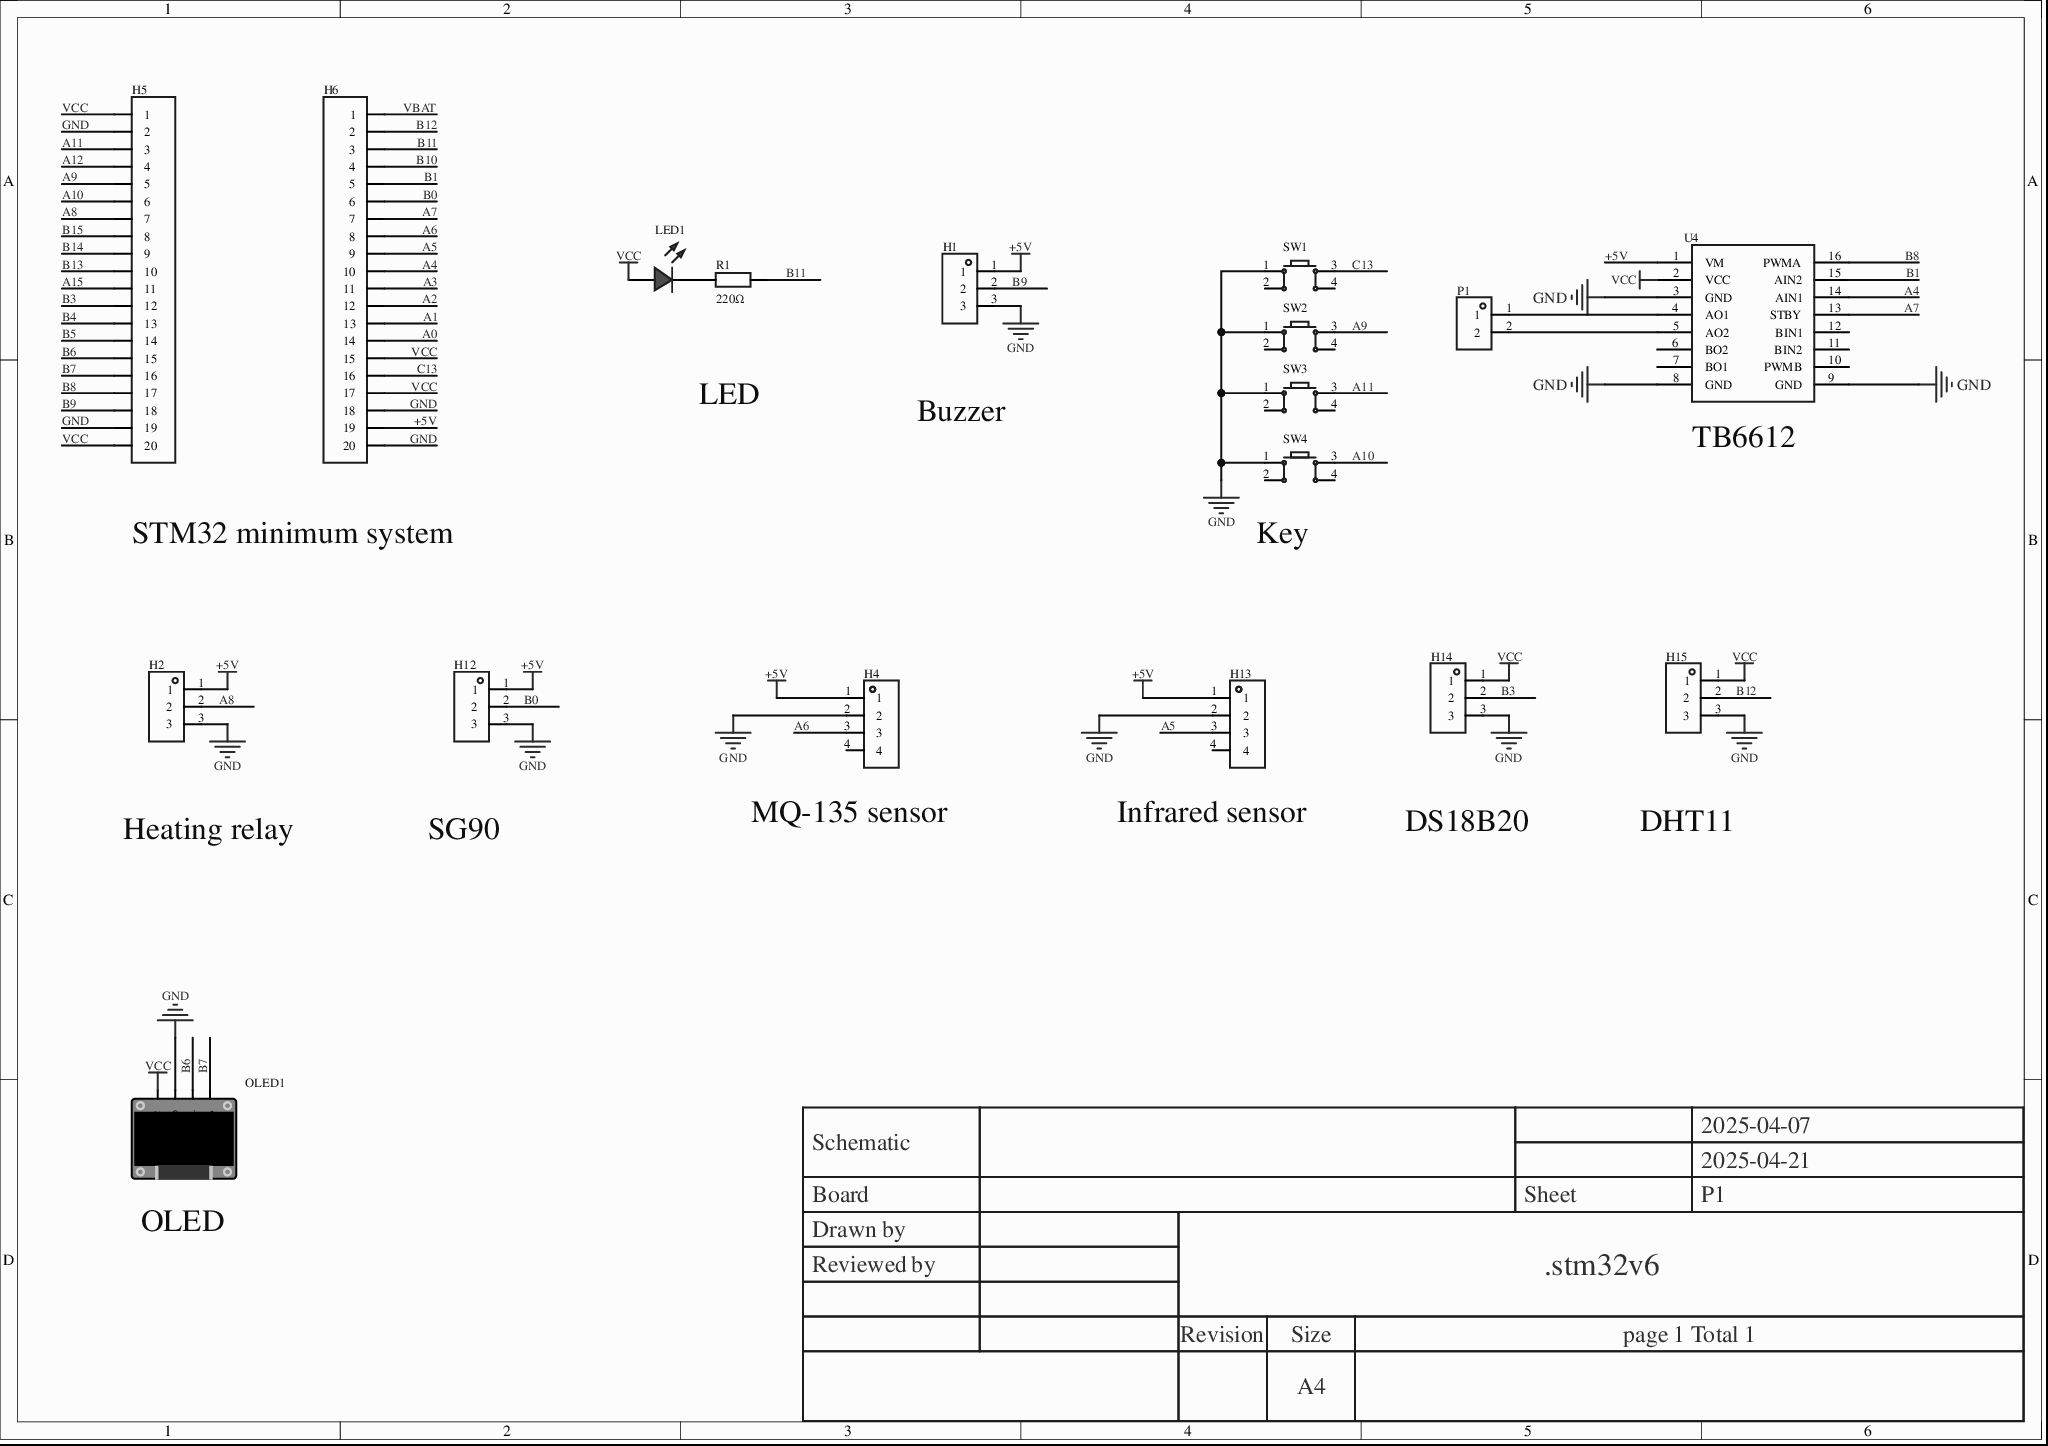
[diagram p0: MISC49946-3.schdoc]
# Altium project MISC49946-2.PrjPcb
1 sheet, 18 parts. Net scope: global (net labels, ports and power ports of the same name join across sheets).
Board file: MISC49946.pcbdoc

## Sheet MISC49946-3.schdoc
size 297 x 209 mm; Version: V1.0; @Project Name: MISC49946; @Page Count: 1; @Update Date: 2026-05-06; @Create Date: 2026-05-06; @Schematic Name: MISC49946; @Page No: 1; @Create Time: 23:22:16; @Update Time: 17:32:40; @Board Name: MISC49946

### Parts
H1  (no value)  [HDR-TH_3P-P2.54-V-F]
H2  (no value)  [HDR-TH_3P-P2.54-V-F]
H4  (no value)  [HDR-TH_4P-P2.54-V-F]
H5  (no value)  [HDR-TH_20P-P2.54-V-F]
H6  (no value)  [HDR-TH_20P-P2.54-V-F]
H12  (no value)  [HDR-TH_3P-P2.54-V-F]
H13  (no value)  [HDR-TH_4P-P2.54-V-F]
H14  (no value)  [HDR-TH_3P-P2.54-V-F]
H15  (no value)  [HDR-TH_3P-P2.54-V-F]
LED1  (no value)  [LED_TH-3mm]
OLED1  (no value)  [0.96OLED_4P]
P1  KF301-2P terminal block  [CONN-TH_XY301V-A-5.0-2P]  (value not drawn)
R1  220Ω  [Res_1/8W]
SW1  (no value)  [SW-TH_4P-L6.0-W6.0-P4.50-LS6.5]
SW2  (no value)  [SW-TH_4P-L6.0-W6.0-P4.50-LS6.5]
SW3  (no value)  [SW-TH_4P-L6.0-W6.0-P4.50-LS6.5]
SW4  (no value)  [SW-TH_4P-L6.0-W6.0-P4.50-LS6.5]
U4  (no value)  [tb6612]

### Nets
+5V: H1.1 H2.1 H4.1 H6.19 H12.1 H13.1 U4.1(VM)
GND: H1.3 H2.3 H4.2 H5.2 H5.19 H6.18 H6.20 H12.3 H13.2 H14.3 H15.3 OLED1.2(GND) SW1.1 SW2.1 SW3.1 SW4.1 U4.3(GND) U4.8(GND) U4.9(GND)
VCC: H5.1 H5.20 H6.15 H6.17 H14.1 H15.1 LED1.1(C) OLED1.1(VCC) U4.2(VCC)
A0: H6.14
A1: H6.13
A2: H6.12
A3: H6.11
A4: H6.10 U4.14(AIN1)
A5: H6.9 H13.3
A6: H4.3 H6.8
A7: H6.7 U4.13(STBY)
A8: H2.2 H5.7
A9: H5.5 SW2.3
A10: H5.6 SW4.3
A11: H5.3 SW3.3
A12: H5.4
A15: H5.11
B0: H6.6 H12.2
B1: H6.5 U4.15(AIN2)
B3: H5.12 H14.2
B4: H5.13
B5: H5.14
B6: H5.15 OLED1.3(SCL)
B7: H5.16 OLED1.4(SDA)
B8: H5.17 U4.16(PWMA)
B9: H1.2 H5.18
B10: H6.4
B11: H6.3 R1.2
B12: H6.2 H15.2
B13: H5.10
B14: H5.9
B15: H5.8
C13: H6.16 SW1.3
VBAT: H6.1
NetLED1_2: LED1.2(A) R1.1
NetP1_1: P1.1 U4.4(AO1)
NetP1_2: P1.2 U4.5(AO2)

Not connected (* = marked no-connect by the designer): H4 4; H13 4; SW1 2 4; SW2 2 4; SW3 2 4; SW4 2 4; U4 6(BO2) 7(BO1) 10(PWMB) 11(BIN2) 12(BIN1)

### Notes on the sheet
- LED
- Buzzer
- (near U4) TB6612
- STM32 minimum system
- (near SW4) Key
- Heating relay
- SG90
- (near H4) MQ-135 sensor
- (near H13) Infrared sensor
- DS18B20
- DHT11
- 串口：
  无通信模块
  GPIO:
  LED灯	PB11
  蜂鸣器  PB9
  按键：	PC13，PA9，PA11，PA10
  加热继电器 PA8
  SG90舵机 PB0
  MQ135空气质量传感器 AO口不接，DO接PA6
  红外AO不接，DO接PA5
  DS18B20   PB3
  DHT11    PB12
  TB6612FNG电机驱动 AO1接有刷小马达+风扇叶正极，AO2接负，PWMA接PB8，AIN2接PB1，AIN1接PA4，STBY接PA7
  IIC:
  0.96英寸OLED显示屏	SDA接PB7 ，SCL接PB6
- OLED
- 2025-04-07
- Schematic
- Board
- Sheet
- 2025-04-21
- P1
- Drawn by
- Reviewed by
- .stm32v6
- Revision
- Size
- A4
- page 1 Total 1

### Library data of the parts
H1 H2 H12 H14 H15 = HDR-F_2.54_1x3P: Symbol: PM254V-11-03-H85; 3D Model: f3b3cc5aae9641bf9e56fc160cef875b; 3D Model Transform: 299.9994,100,0,0,0,0,0,0,-118.11; ConvertToPcb: yes; ModelName: HDR2.54-F-LI-1X3P; Device: HDR-F_2.54_1x3P; Supplier Part: C541850; Supplier Footprint: 插件; FootprintName: HDR-TH_3P-P2.54-V-F; AddInBom: yes
H4 = HDR-F_2.54_1x4P: Symbol: 2.54-1*4P female; ConvertToPcb: yes; ModelId: d187812051054f85879fcaa51a310d8e0819f05c4eef4c71ace90d822a990e87; ModelTransform: 419.6842,98.464,0,0,0,0,0,0,-118.11; Device: HDR-F_2.54_1x4P; FootprintName: HDR-TH_4P-P2.54-V-F; AddInBom: yes; SupplierPart: C2718488; Supplier Footprint: 插件; ModelName: HDR-TH_4P-P2.54-V-F
H5 H6 = HDR-F_2.54_1x20P: ConvertToPcb: yes; ModelId: db7015f7ad9d48b8a3b1188db02e3429; ModelName: HDR-F-2.54_1x20; ModelTransform: 1999.996,100,0,0,0,0,0,0,-118.11; Symbol: HDR-F_2.54_1x20P; Device: HDR-F_2.54_1x20P; AddInBom: yes; SupplierPart: C50984; Supplier Footprint: 插件; FootprintName: HDR-TH_20P-P2.54-V-F
H13 = HDR-F_2.54_1x4P: Symbol: 2.54-1*4P female; 3D Model: d187812051054f85879fcaa51a310d8e0819f05c4eef4c71ace90d822a990e87; 3D Model Transform: 419.6842,98.464,0,0,0,0,0,0,-118.11; ConvertToPcb: yes; Device: HDR-F_2.54_1x4P; Supplier Part: C2718488; Supplier Footprint: 插件; FootprintName: HDR-TH_4P-P2.54-V-F; AddInBom: yes; ModelName: HDR-TH_4P-P2.54-V-F
LED1 = LED_TH-R_3mm: ConvertToPcb: yes; ModelId: a497c992633541038a38947cdc58012f0819f05c4eef4c71ace90d822a990e87; ModelName: LED-TH-3mm_R; ModelTransform: 141.274,153.327,0,0,0,0,-5.984,0,-137.795; Symbol: LED_TH-R; Device: LED_TH-R_3mm; AddInBom: yes; FootprintName: LED_TH-3mm; Supplier Footprint: 插件
OLED1 = 0.96OLED模块_4P: Symbol: 0.96OLED module_4P_1; Device: 0.96OLED module_4P; ConvertToPcb: yes; ModelId: 79c000fdb68d45a296c2e9bedf4f9055; ModelTransform: 1393.69792,1318.895,0,0,0,0,0,-560.079,-137.795; AddInBom: yes; FootprintName: 0.96OLED_4P; Supplier Footprint: 插件; ModelName: 0.96OLED_4P
P1 = KF301-2P接线端子: 3D Model: ef7ead88b0f2448d904975b26718870f; 3D Model Transform: 417.322,299.212,0,0,0,0,11.811,-7.835,-157.48; AddInBom: yes; Symbol: KF301-2P terminal block; Device: KF301-2P terminal block; LCSC Part Name: KF301-2P接线端子; Supplier Part: C9900016950; Manufacturer Part: KF301-2P接线端子; Supplier Footprint: CK301-2P; Supplier: LCSC; ConvertToPcb: yes; FootprintName: CONN-TH_XY301V-A-5.0-2P; ModelName: CONN-TH_XY301V-A-5.0-2P
R1 = Res_AXIAL-1/8W: Symbol: Resistor; ConvertToPcb: yes; ModelId: b2b5ae7ae4c642178fe0039925c86a3f0819f05c4eef4c71ace90d822a990e87; ModelName: RES-TH_BD1.8-L3.2-P7.20-D0.4; ModelTransform: 282.86,66.88,253.09,0,0,0,0,0,-191; Device: Res_AXIAL-1/8W; Value: 220Ω; AddInBom: yes; Supplier Footprint: 轴向引线; FootprintName: Res_1/8W
SW1-SW4 = Key_TH_6x6x6: Contact current:50mA; Rated voltage (DC):12V; Insulation resistance:100MΩ; Circuit structure: single pole single throw; Mounting: through-hole; Button shape: round button; Button/cap colour: black; Operating force: 260gf@±30gf; Operating temperature: -25℃~+70℃; Pin style: PC pin; Switch length: 6mm; Switch width: 6mm; Switch height: 6mm; With bracket: no;; Symbol: Tactile push button; AddInBom: yes; ModelId: 20eee248bc684ccd8cbdbb1d0d91ec6f0819f05c4eef4c71ace90d822a990e87; ModelName: SW-TH_4P-L6.0-W6.0-H5.0-LS6.5-P4.50; ModelTransform: 236.22,323.03,0,90,0,0,0,0,-137.795; Device: Key_TH_6x6x6; FootprintName: SW-TH_4P-L6.0-W6.0-P4.50-LS6.5; ConvertToPcb: yes; Supplier Footprint: 插件
U4 = tb6612: AddInBom: yes; Symbol: tb6612; Device: tb6612; JLCPCB Part Class: Extended library; ConvertToPcb: yes; FootprintName: tb6612